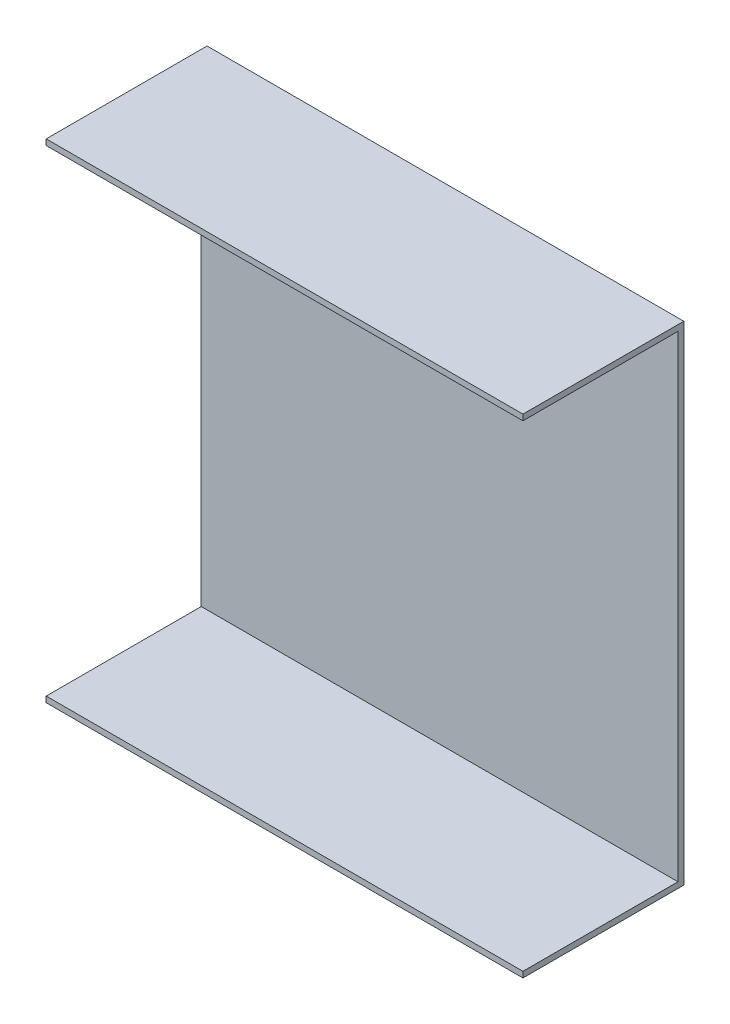
SolidWorks part; units mm, degrees
ref_plane "Front Plane" through (0, 0, 0) normal (0, 0, 1) x (1, 0, 0)
ref_plane "Top Plane" through (0, 0, 0) normal (0, 1, 0) x (1, 0, 0)
ref_plane "Right Plane" through (0, 0, 0) normal (1, 0, 0) x (0, 0, -1)
sketch "Sketch1" plane through (0, 0, 0) normal (0, 0, 1) x (1, 0, 0)
  line L1 (-123, 126) -> (123, 126)
  line L2 (-123, 126) -> (-123, -126)
  line L3 (-123, -126) -> (123, -126)
  line L4 (123, 126) -> (123, -126)
  line L5 (-123, 126) -> (123, -126) construction
  line L6 (-123, -126) -> (123, 126) construction
  point P0 (0, 0)
  dimension "D1" = 246
  dimension "D2" = 252
extrude "Boss-Extrude1" add sketch "Sketch1" along normal blind 3
sketch "Sketch2" plane through (0, 0, 3) normal (0, 0, 1) x (1, 0, 0)
  line L0 (123, -126) -> (123, 126) construction
  line L1 (-123, 126) -> (123, 126)
  line L2 (-123, 126) -> (-123, 123)
  line L3 (-123, 123) -> (123, 123)
  line L4 (123, 126) -> (123, 123)
  line L5 (-123, 126) -> (-123, -126) construction
  line L6 (123, -126) -> (-123, -126)
  line L7 (123, -126) -> (123, -123)
  line L8 (123, -123) -> (-123, -123)
  line L9 (-123, -126) -> (-123, -123)
  dimension "D1" = 3
  dimension "D2" = 3
extrude "Boss-Extrude2" add sketch "Sketch2" along normal blind 80
